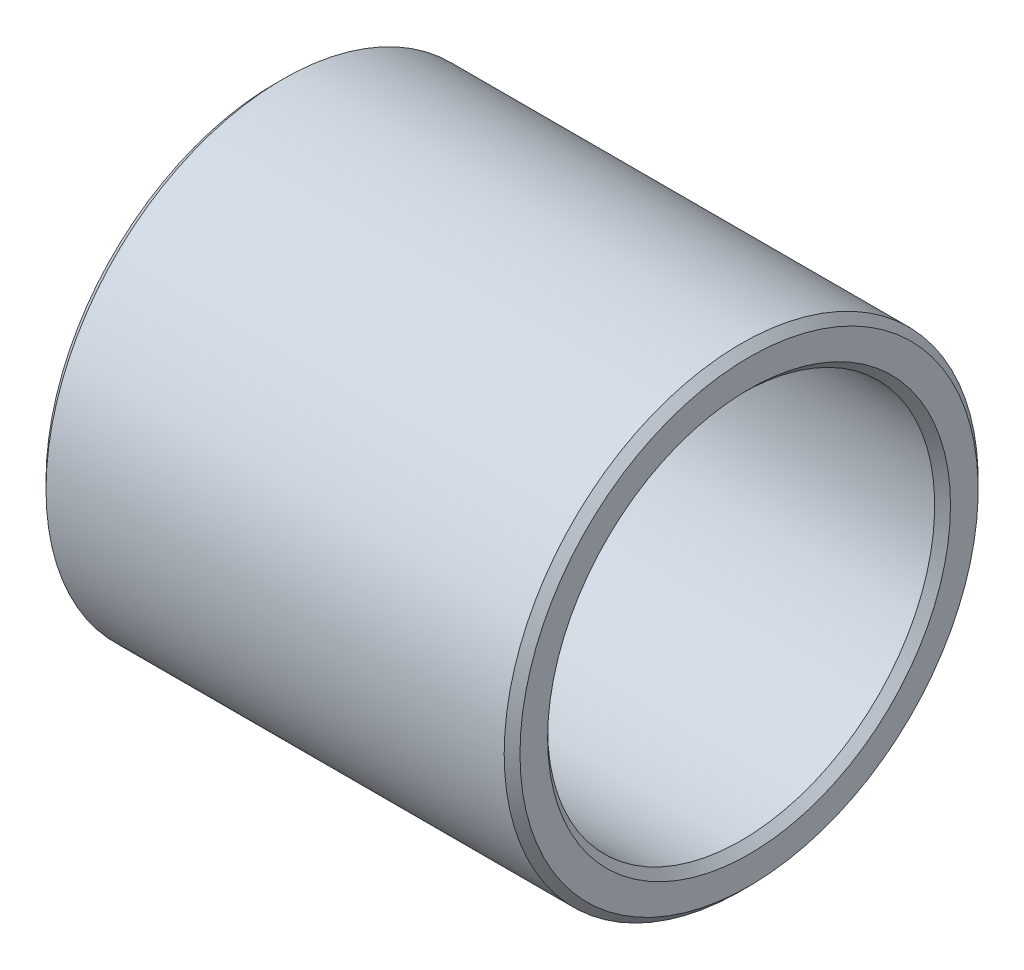
from build123d import *


with BuildPart() as part:
    # 草图1 → 旋转1 (revolve)
    with BuildSketch(Plane(origin=(0, 0, 0), x_dir=(1, 0, 0), z_dir=(0, 1, 0)), mode=Mode.PRIVATE) as revolve_1_sk:
        Polygon((-15, 14.5), (-14.5, 15), (14.5, 15), (15, 14.5), (15, 12.75), (14.5, 12.25), (-14.5, 12.25), (-15, 12.75), align=None)
    revolve(revolve_1_sk.sketch.rotate(Axis((-1000, 0, 0), (1, 0, 0)), 180), axis=Axis((-1000, 0, 0), (1, 0, 0)))


solid = part.part
